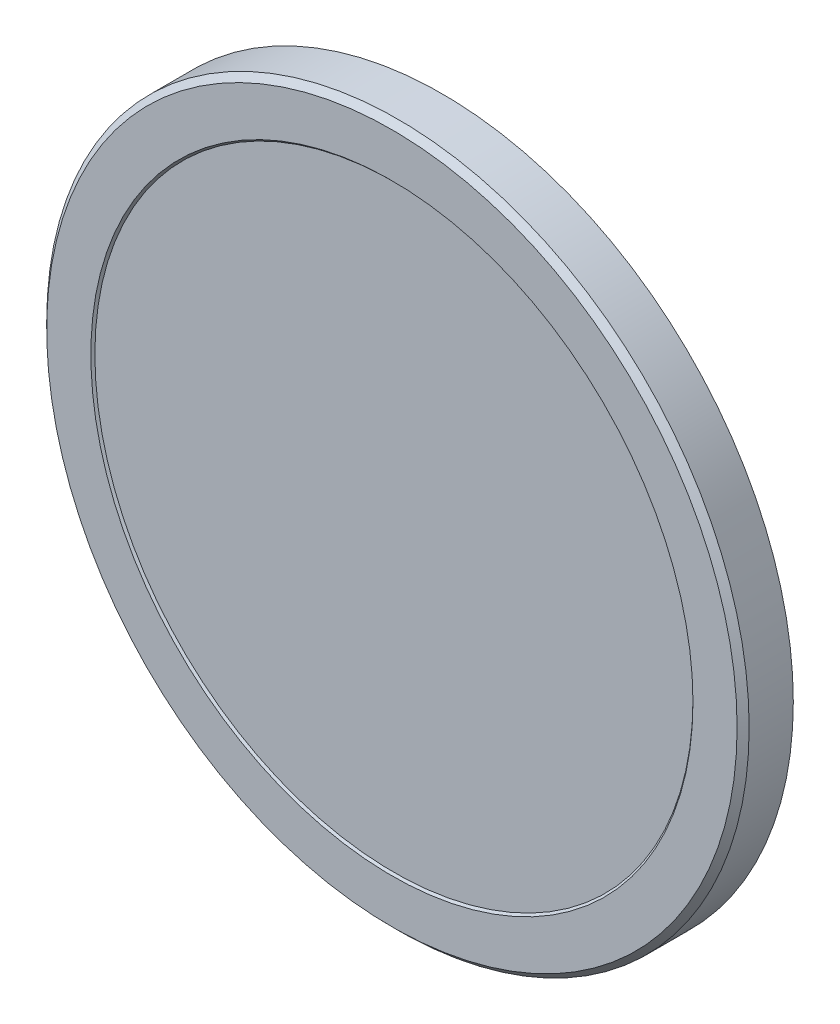
from build123d import *

# Parameters (mm, degrees)
SKETCH1_R           = 34
BOSS_EXTRUDE1_DEPTH = 50
SKETCH2_R           = 175
BOSS_EXTRUDE2_DEPTH = 25
SKETCH3_R           = 150
CUT_EXTRUDE1_DEPTH  = 1
CUT_EXTRUDE1_DRAFT  = -45
FILLET1_R           = 0.5
CHAMFER1_SIZE       = 3


with BuildPart() as part:
    # Sketch1 → Boss-Extrude1 (new body)
    with BuildSketch(Plane.XY):
        Circle(SKETCH1_R)
    extrude(amount=BOSS_EXTRUDE1_DEPTH)

    # Sketch2 → Boss-Extrude2 (add)
    with BuildSketch(Plane.XY.offset(50)):
        Circle(SKETCH2_R)
    extrude(amount=-BOSS_EXTRUDE2_DEPTH)


with BuildPart() as cut_extrude1_tool:
    # Sketch3 → Cut-Extrude1 (with draft: the straight prism first)
    with BuildSketch(Plane.XY.offset(50)):
        Circle(SKETCH3_R)
    extrude(amount=-CUT_EXTRUDE1_DEPTH)
    # Cut-Extrude1: the draft: its side faces are tilted about the plane it starts from
    cut_extrude1_sides = [cut_extrude1_tool.faces().sort_by_distance(p)[0] for p in [
        (-150, 0, 49.5),
    ]]
    draft(cut_extrude1_sides, Plane.XY.offset(50), CUT_EXTRUDE1_DRAFT)


with BuildPart() as part_1:
    add(part.part)

    # Cut-Extrude1: cut by cut_extrude1_tool
    add(cut_extrude1_tool.part, mode=Mode.SUBTRACT)

    # Fillet1
    fillet1_edges = [part_1.edges().sort_by_distance(p)[0] for p in [
        (-34, 0, 25),
    ]]
    fillet(fillet1_edges, radius=FILLET1_R)

    # Chamfer1
    chamfer1_edges = [part_1.edges().sort_by_distance(p)[0] for p in [
        (-175, 0, 50),
    ]]
    chamfer(chamfer1_edges, length=CHAMFER1_SIZE)


solid = part_1.part
